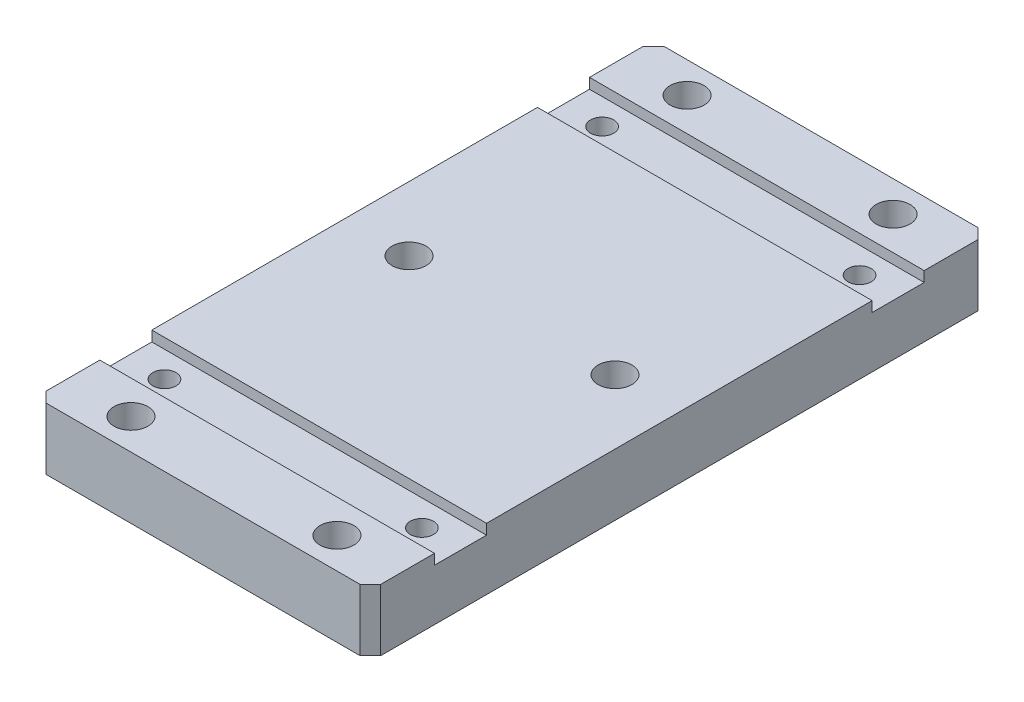
from build123d import *

# Parameters (mm, degrees)
SKETCH_1_W                   = 65
SKETCH_1_H                   = 120
EXTRUDE_1_DEPTH              = 12
HOLE_WIZARD_M6_1_D           = 6.6
SKETCH_4_W                   = 65
SKETCH_4_H                   = 10.1
CUT_EXTRUDE_1_DEPTH          = 2
CHAMFER_1_SIZE               = 2
HOLE_WIZARD_M4_1_D           = 4.5
HOLE_WIZARD_M4_1_CBORE_D     = 8
HOLE_WIZARD_M4_1_CBORE_DEPTH = 4.6


with BuildPart() as part:
    # 草图1 → 凸台-拉伸1 (new body)
    with BuildSketch(Plane(origin=(0, 0, 0), x_dir=(1, 0, 0), z_dir=(0, 1, 0))):
        Rectangle(SKETCH_1_W, SKETCH_1_H)
    extrude(amount=EXTRUDE_1_DEPTH)

    # M6 间隙孔1 (through all)
    with Locations(Plane(origin=(0, 12, 0), x_dir=(1, 0, 0), z_dir=(0, 1, 0))):
        with Locations((-20, -54), (20, -54), (-20, 0), (20, 0), (-20, 54), (20, 54)):
            Hole(HOLE_WIZARD_M6_1_D / 2)

    # 草图4 → 切除-拉伸1 (cut)
    with BuildSketch(Plane(origin=(0, 12, 0), x_dir=(1, 0, 0), z_dir=(0, 1, 0))):
        with Locations((0, 42.5)):
            Rectangle(SKETCH_4_W, SKETCH_4_H)
        with Locations((0, -42.5)):
            Rectangle(SKETCH_4_W, SKETCH_4_H)
    extrude(amount=-CUT_EXTRUDE_1_DEPTH, mode=Mode.SUBTRACT)

    # 倒角1
    chamfer_1_edges = [part.edges().sort_by_distance(p)[0] for p in [
        (32.5, 6, 60),
        (-32.5, 6, 60),
        (-32.5, 6, -60),
        (32.5, 6, -60),
    ]]
    chamfer(chamfer_1_edges, length=CHAMFER_1_SIZE)

    # M4 六角圆柱头螺钉的柱形沉头孔1 (through all)
    with Locations(Plane(origin=(0, 0, 0), x_dir=(-1, 0, 0), z_dir=(0, -1, 0))):
        with Locations((-25, 42.5), (-25, -42.5), (25, -42.5), (25, 42.5)):
            CounterBoreHole(HOLE_WIZARD_M4_1_D / 2, HOLE_WIZARD_M4_1_CBORE_D / 2, HOLE_WIZARD_M4_1_CBORE_DEPTH)


solid = part.part
